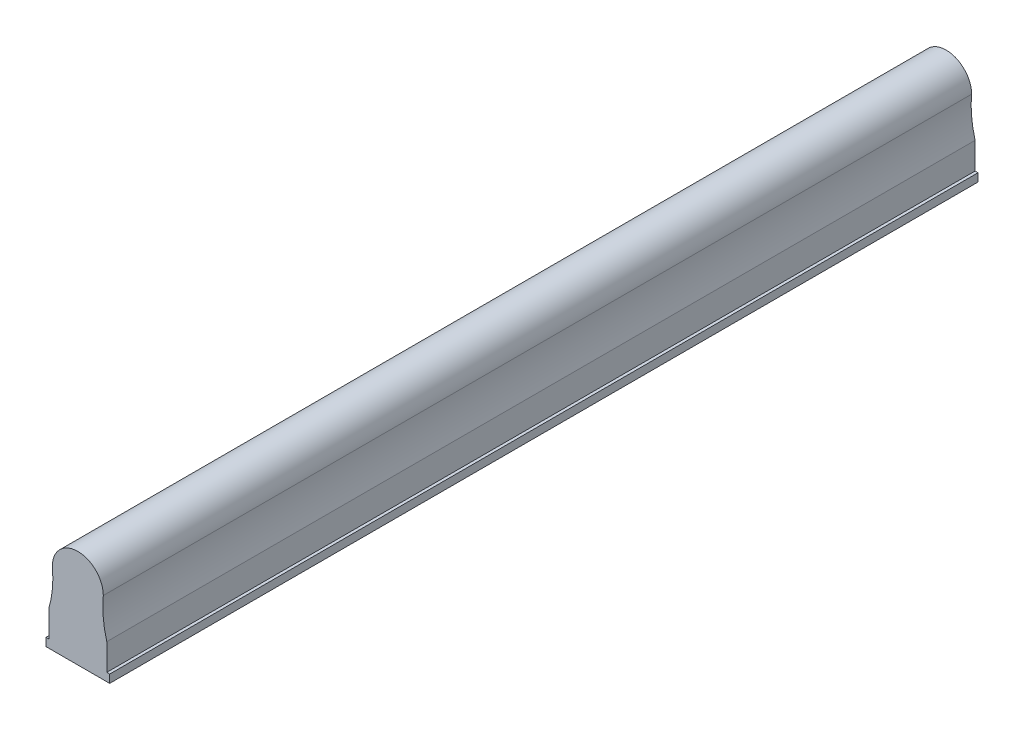
SolidWorks part; units mm, degrees
ref_plane "前视" through (0, 0, 0) normal (0, 0, 1) x (1, 0, 0)
ref_plane "上视" through (0, 0, 0) normal (0, 1, 0) x (1, 0, 0)
ref_plane "右视" through (0, 0, 0) normal (1, 0, 0) x (0, 0, -1)
sketch "草图1" plane through (0, 0, 0) normal (0, 0, 1) x (1, 0, 0)
  line L0 (0, 0) -> (38.21, 0) construction
  line L1 (0, 0) -> (0, 45.5378) construction
  line L2 (0, 34) -> (-19.5553, 34) construction
  line L3 (10, 12) -> (10, 2.8)
  line L4 (10, 2.8) -> (11, 2.8)
  line L5 (11, 2.8) -> (11, 0)
  line L6 (11, 0) -> (-11, 0)
  line L7 (-11, 2.8) -> (-11, 0)
  line L8 (-10, 2.8) -> (-11, 2.8)
  line L9 (-10, 12) -> (-10, 2.8)
  arc A0 (8.8, 25.2) -> (-8.8, 25.2) centre (0, 25.2) ccw
  spline S0 degree 2 poles (8.8, 25.2) (8.1482, 18.4837) (10, 12) knots 0 0 0 1 1 1
  spline S1 degree 2 poles (-8.8, 25.2) (-8.1482, 18.4837) (-10, 12) knots 0 0 0 1 1 1
  dimension "D1" = 17.6
  dimension "D2" = 34
  dimension "D3" = 10
  dimension "D4" = 11
  dimension "D5" = 2.8
  dimension "D6" = 12
extrude "凸台-拉伸1" add sketch "草图1" along normal blind 300
